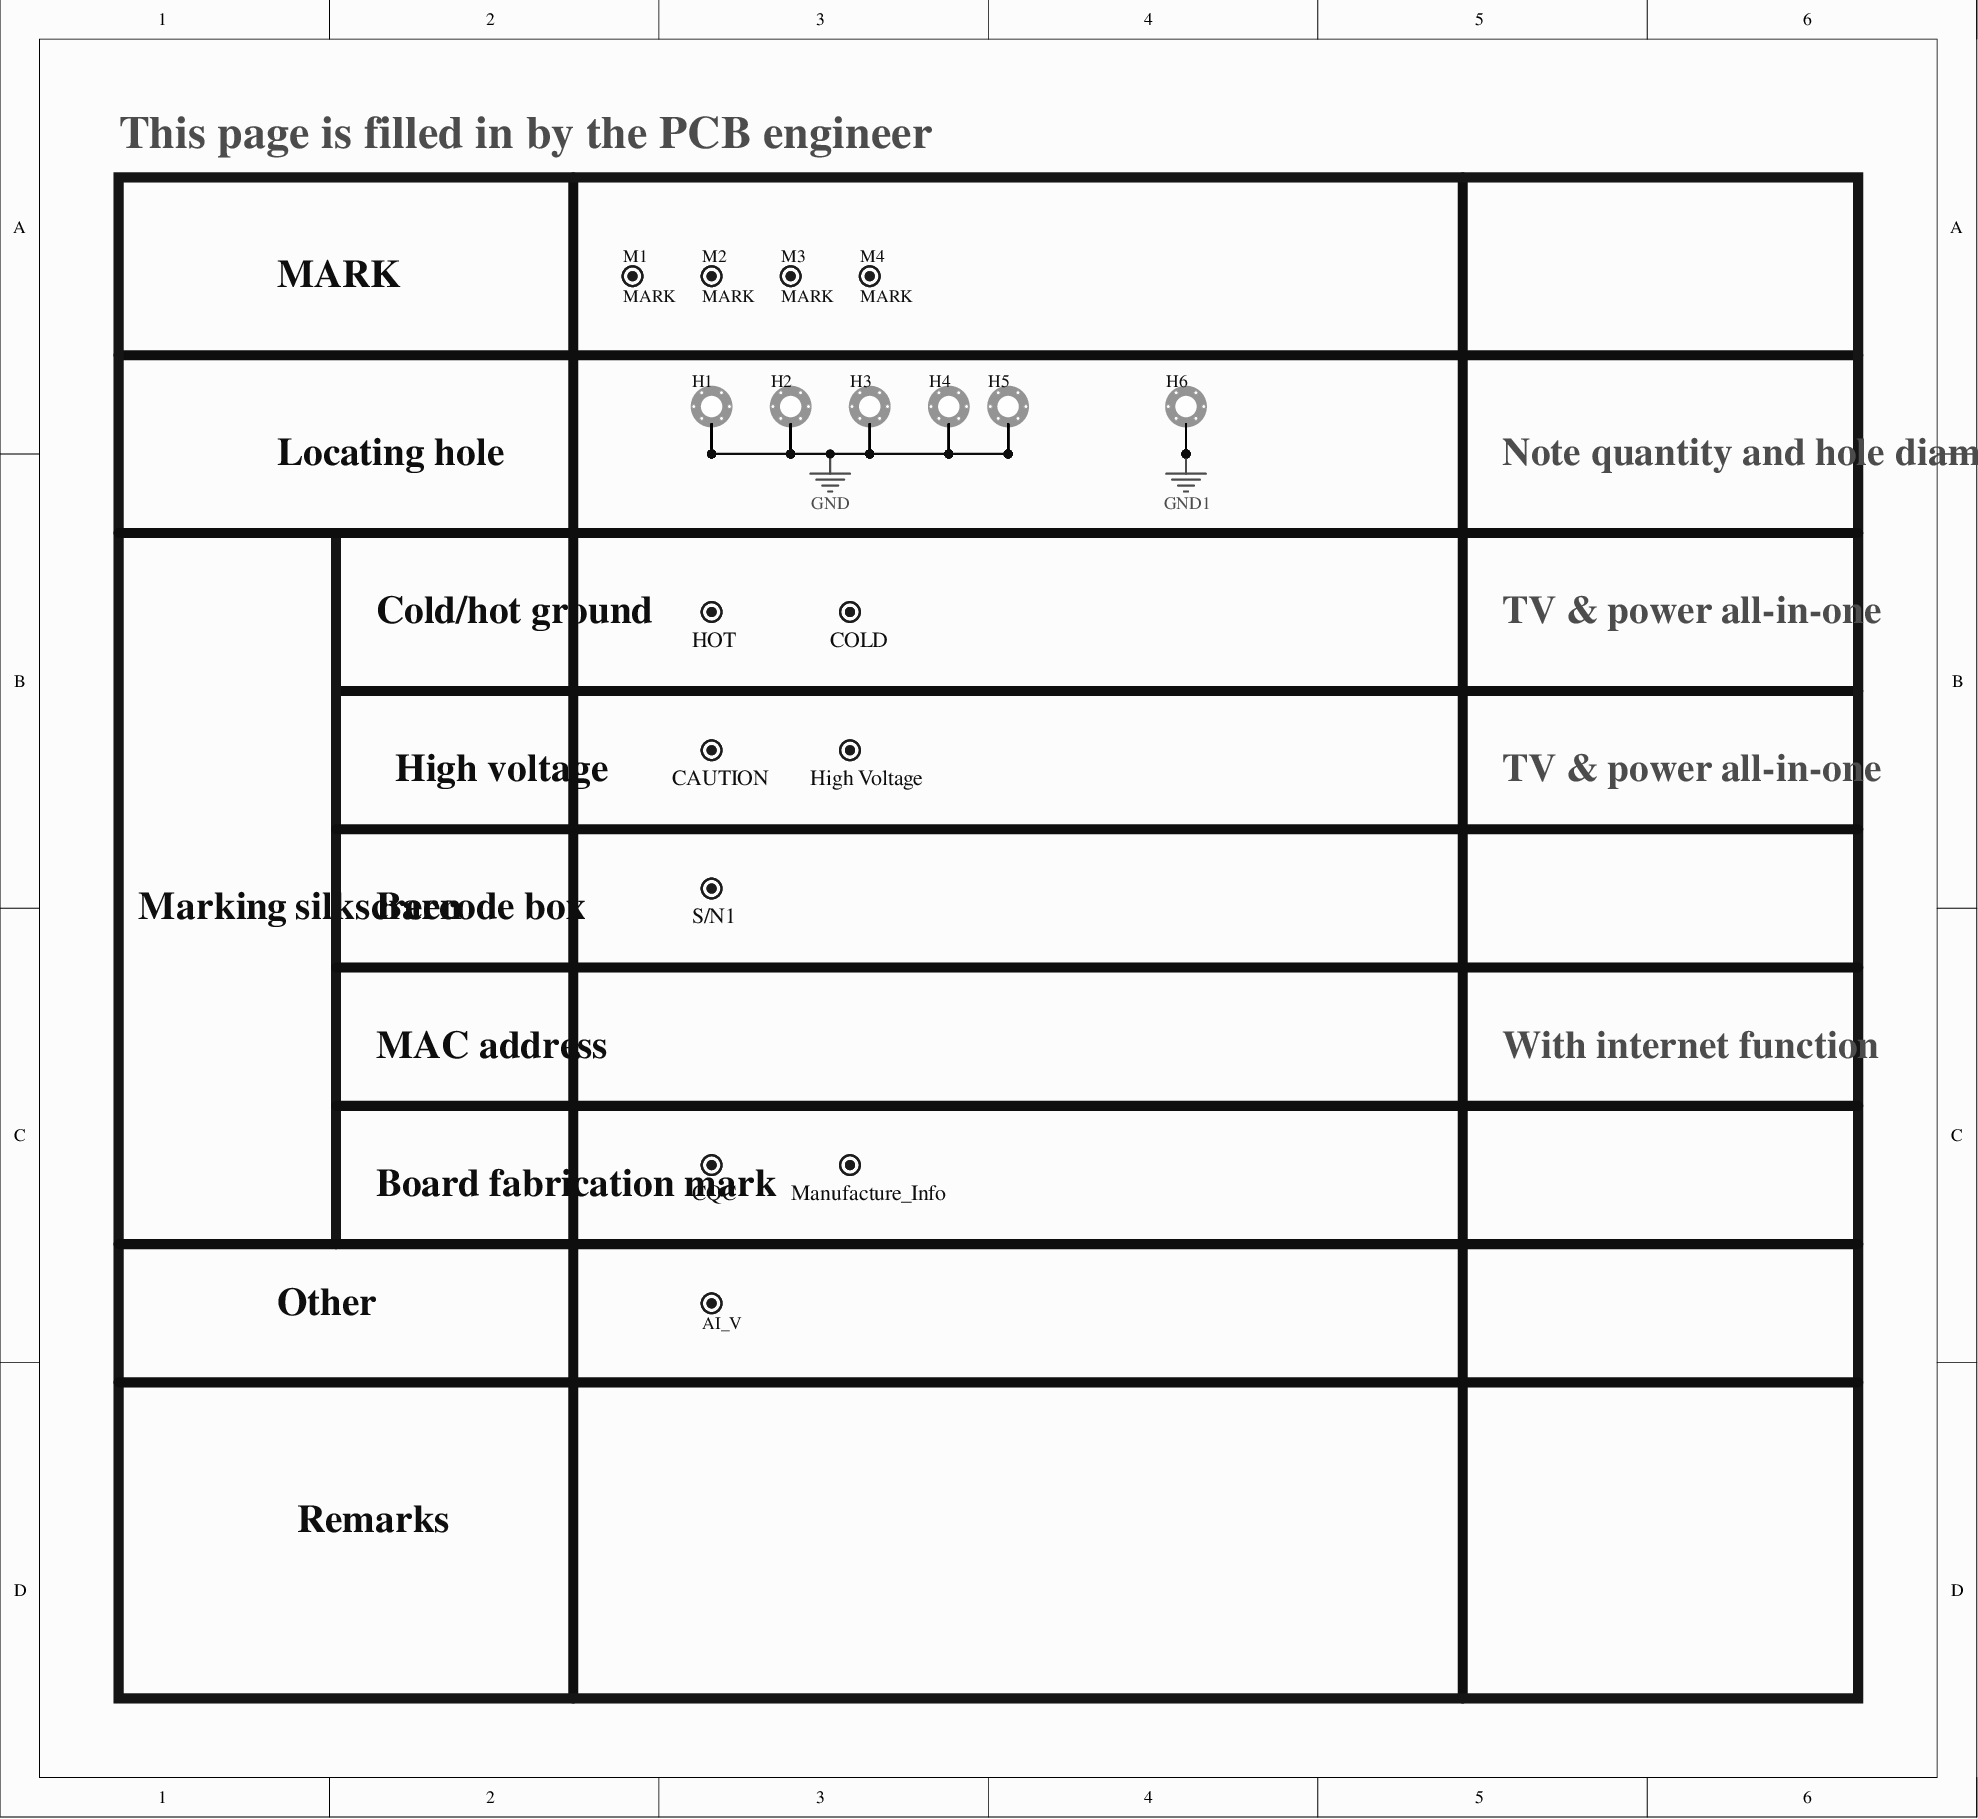
[diagram p0: MISC86372-4.SchDoc]
# Altium project MISC86372-32.PrjPCB (part 1 of 8)
13 sheets, 578 parts. Net scope: global (net labels, ports and power ports of the same name join across sheets).
Board file: MISC86372.PcbDoc
Sheets:
  MISC86372-4.SchDoc
  MISC86372-6.SchDoc
  MISC86372-17.SchDoc
  MISC86372-8.SchDoc
  MISC86372-9.SchDoc
  MISC86372-10.SchDoc
  MISC86372-11.SchDoc
  MISC86372-12.SchDoc
  MISC86372-13.SchDoc
  MISC86372-14.SchDoc
  MISC86372-15.SchDoc
  MISC86372-16.SchDoc
  MISC86372-5.SchDoc

## Sheet MISC86372-4.SchDoc
size 254 x 233 mm

### Parts
AI_V  AI_GRIPPER_V  [AI_GRIPPER_V]  (value not drawn)
CAUTION  CAUTION  [CAUTION]
COLD  COLD  [COLD]
CQC  CQC  [CQC]
H1  Location hole  [ASSE4.0C-3]  (value not drawn)
H2  Location hole  [ASSE3.5C-3]  (value not drawn)
H3  Location hole  [ASSE3.5C-3]  (value not drawn)
H4  Location hole  [ASSE5.0C-3]  (value not drawn)
H5  Location hole  [ASSE3.5C-3]  (value not drawn)
H6  Location hole  [ASSE3.5C-3]  (value not drawn)
High_Voltage  High Voltage  [High Voltage]
HOT  HOT  [HOT]
M1  MARK  [MARK]
M2  MARK  [MARK]
M3  MARK  [MARK]
M4  MARK  [MARK]
Manufacture_Info  Manufacture_Info  [Manufacture_Info]
S/N1  Barcode  [Barcode]  (value not drawn)

### Nets
GND: H1.1 H1.2 H1.3 H1.4 H1.5 H1.6 H2.1 H2.2 H2.3 H2.4 H2.5 H2.6 H3.1 H3.2 H3.3 H3.4 H3.5 H3.6 H4.1 H4.2 H4.3 H4.4 H4.5 H4.6 H5.1 H5.2 H5.3 H5.4 H5.5 H5.6
GND1: H6.1 H6.2 H6.3 H6.4 H6.5 H6.6

### Notes on the sheet
- This page is filled in by the PCB engineer
- MARK
- Locating hole
- Note quantity and hole diameter
- (near HOT) Cold/hot ground
- TV & power all-in-one
- High voltage
- Marking silkscreen
- Barcode box
- MAC address
- With internet function
- (near CQC) Board fabrication mark
- Other
- Remarks

### Library data of the parts
H1-H6 = Location hole-D
M1-M4 = MARK-D

## Sheet MISC86372-6.SchDoc
size 254 x 322 mm
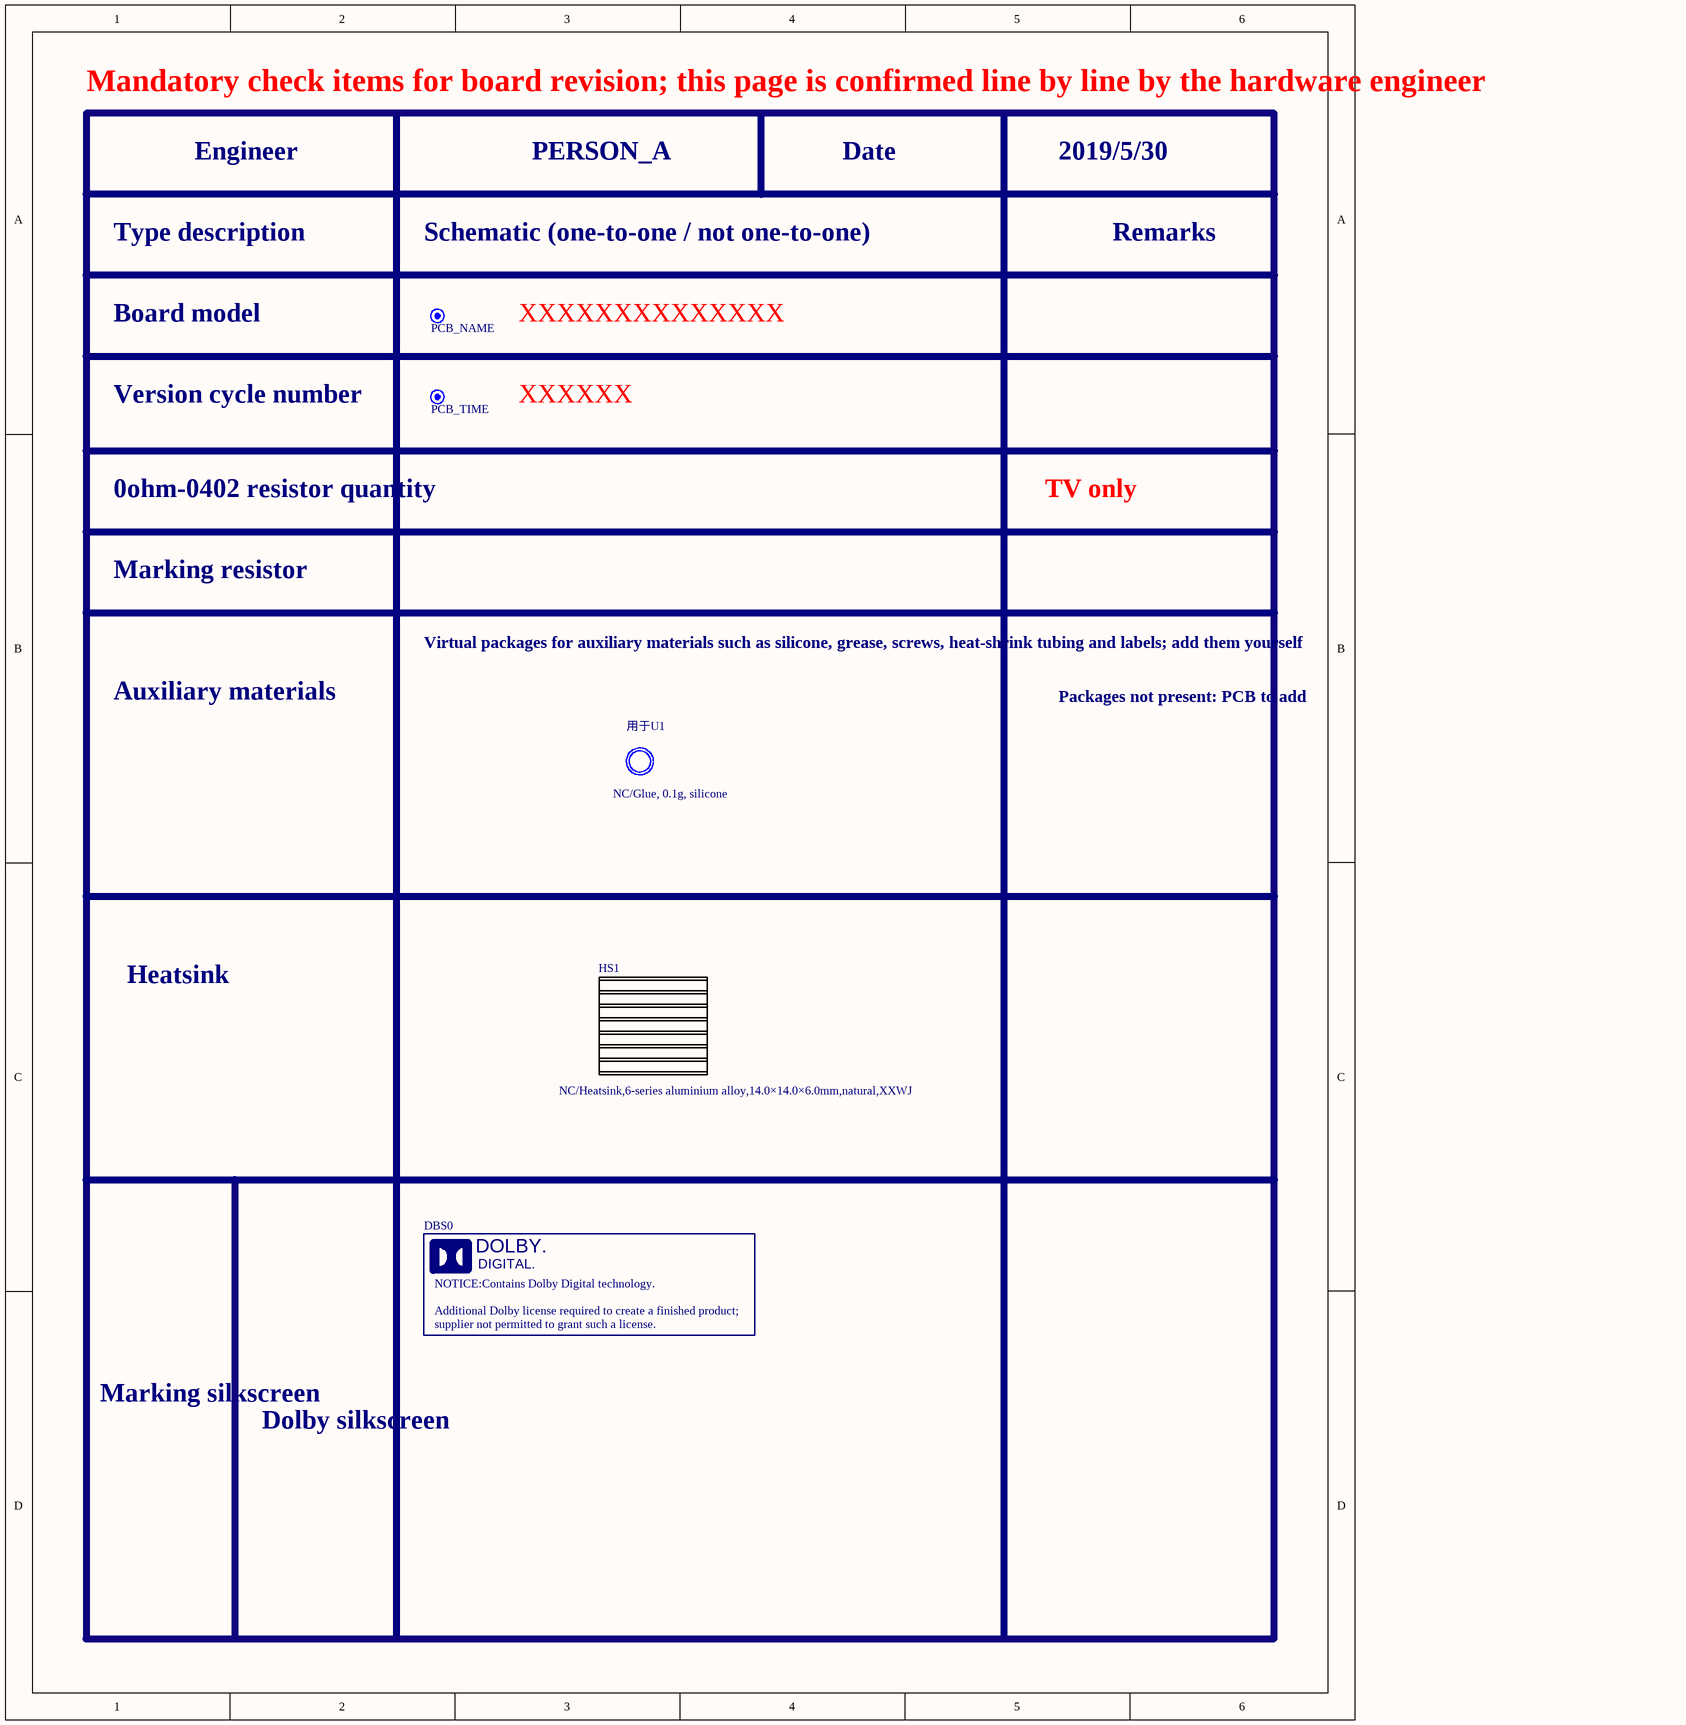
[diagram p1: MISC86372-6.SchDoc]

### Parts
DBS0  DOLBY  [DOLBY-SILK]  (value not drawn)
HS1  NC/Heatsink,6-series aluminium alloy,14.0×14.0×6.0mm,natural,XXWJ  [HS(14*14*6)]
XXXXXX  PCB_TIME  [PCB_TIME]
XXXXXXXXXXXXXX  PCB_NAME  [PCB_NAME]
用于U1  NC/Glue, 0.1g, silicone  [Heat-Shrinkable Tube]

### Notes on the sheet
- Mandatory check items for board revision; this page is confirmed line by line by the hardware engineer
- Engineer
- PERSON_A
- Date
- 2019/5/30
- Type description
- Schematic (one-to-one / not one-to-one)
- Remarks
- Board model
- Version cycle number
- 0ohm-0402 resistor quantity
- TV only
- Marking resistor
- Virtual packages for auxiliary materials such as silicone, grease, screws, heat-shrink tubing and labels; add them yourself
- Auxiliary materials
- Packages not present: PCB to add
- Heatsink
- Marking silkscreen
- Dolby silkscreen

### Library data of the parts
HS1 = 14×14×06-THD-HS: SMD heatsink
用于U1 = Φ12mm×12mm-黑色-125度(UL认证)-D